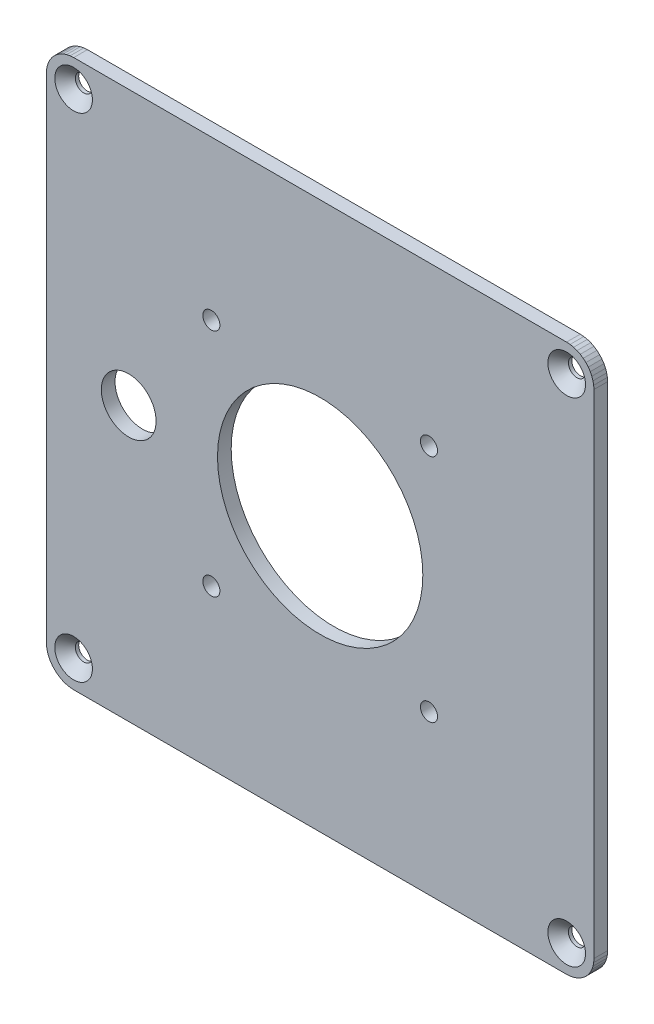
SolidWorks part; units mm, degrees
ref_plane "Front Plane" through (0, 0, 0) normal (0, 0, 1) x (1, 0, 0)
ref_plane "Top Plane" through (0, 0, 0) normal (0, 1, 0) x (1, 0, 0)
ref_plane "Right Plane" through (0, 0, 0) normal (1, 0, 0) x (0, 0, -1)
ref_plane "Plane1" through (0, 0, 196.7768) normal (0, 0, 1) x (1, 0, 0)
sketch "Sketch1" plane through (0, 0, 196.7768) normal (0, 0, 1) x (1, 0, 0)
  line L0 (-40, -36) -> (-39.9658, -36.5221)
  line L1 (-39.9658, -36.5221) -> (-39.8637, -37.0353)
  line L2 (-39.8637, -37.0353) -> (-39.6955, -37.5307)
  line L3 (-39.6955, -37.5307) -> (-39.4641, -38)
  line L4 (-39.4641, -38) -> (-39.1734, -38.435)
  line L5 (-39.1734, -38.435) -> (-38.8284, -38.8284)
  line L6 (-38.8284, -38.8284) -> (-38.435, -39.1734)
  line L7 (-38.435, -39.1734) -> (-38, -39.4641)
  line L8 (-38, -39.4641) -> (-37.5307, -39.6955)
  line L9 (-37.5307, -39.6955) -> (-37.0353, -39.8637)
  line L10 (-37.0353, -39.8637) -> (-36.5221, -39.9658)
  line L11 (-36.5221, -39.9658) -> (-36, -40)
  line L12 (-36, -40) -> (36, -40)
  line L13 (36, -40) -> (36.5221, -39.9658)
  line L14 (36.5221, -39.9658) -> (37.0353, -39.8637)
  line L15 (37.0353, -39.8637) -> (37.5307, -39.6955)
  line L16 (37.5307, -39.6955) -> (38, -39.4641)
  line L17 (38, -39.4641) -> (38.435, -39.1734)
  line L18 (38.435, -39.1734) -> (38.8284, -38.8284)
  line L19 (38.8284, -38.8284) -> (39.1734, -38.435)
  line L20 (39.1734, -38.435) -> (39.4641, -38)
  line L21 (39.4641, -38) -> (39.6955, -37.5307)
  line L22 (39.6955, -37.5307) -> (39.8637, -37.0353)
  line L23 (39.8637, -37.0353) -> (39.9658, -36.5221)
  line L24 (39.9658, -36.5221) -> (40, -36)
  line L25 (40, -36) -> (40, 36)
  line L26 (40, 36) -> (39.9658, 36.5221)
  line L27 (39.9658, 36.5221) -> (39.8637, 37.0353)
  line L28 (39.8637, 37.0353) -> (39.6955, 37.5307)
  line L29 (39.6955, 37.5307) -> (39.4641, 38)
  line L30 (39.4641, 38) -> (39.1734, 38.435)
  line L31 (39.1734, 38.435) -> (38.8284, 38.8284)
  line L32 (38.8284, 38.8284) -> (38.435, 39.1734)
  line L33 (38.435, 39.1734) -> (38, 39.4641)
  line L34 (38, 39.4641) -> (37.5307, 39.6955)
  line L35 (37.5307, 39.6955) -> (37.0353, 39.8637)
  line L36 (37.0353, 39.8637) -> (36.5221, 39.9658)
  line L37 (36.5221, 39.9658) -> (36, 40)
  line L38 (36, 40) -> (-36, 40)
  line L39 (-36, 40) -> (-36.5221, 39.9658)
  line L40 (-36.5221, 39.9658) -> (-37.0353, 39.8637)
  line L41 (-37.0353, 39.8637) -> (-37.5307, 39.6955)
  line L42 (-37.5307, 39.6955) -> (-38, 39.4641)
  line L43 (-38, 39.4641) -> (-38.435, 39.1734)
  line L44 (-38.435, 39.1734) -> (-38.8284, 38.8284)
  line L45 (-38.8284, 38.8284) -> (-39.1734, 38.435)
  line L46 (-39.1734, 38.435) -> (-39.4641, 38)
  line L47 (-39.4641, 38) -> (-39.6955, 37.5307)
  line L48 (-39.6955, 37.5307) -> (-39.8637, 37.0353)
  line L49 (-39.8637, 37.0353) -> (-39.9658, 36.5221)
  line L50 (-39.9658, 36.5221) -> (-40, 36)
  line L51 (-40, 36) -> (-40, -36)
  line L52 (-37.4489, -36.3882) -> (-37.5, -36)
  line L53 (-37.5, -36) -> (-37.4489, -35.6118)
  line L54 (-37.4489, -35.6118) -> (-37.299, -35.25)
  line L55 (-37.299, -35.25) -> (-37.0607, -34.9393)
  line L56 (-37.0607, -34.9393) -> (-36.75, -34.701)
  line L57 (-36.75, -34.701) -> (-36.3882, -34.5511)
  line L58 (-36.3882, -34.5511) -> (-36, -34.5)
  line L59 (-36, -34.5) -> (-35.6118, -34.5511)
  line L60 (-35.6118, -34.5511) -> (-35.25, -34.701)
  line L61 (-35.25, -34.701) -> (-34.9393, -34.9393)
  line L62 (-34.9393, -34.9393) -> (-34.701, -35.25)
  line L63 (-34.701, -35.25) -> (-34.5511, -35.6118)
  line L64 (-34.5511, -35.6118) -> (-34.5, -36)
  line L65 (-34.5, -36) -> (-34.5511, -36.3882)
  line L66 (-34.5511, -36.3882) -> (-34.701, -36.75)
  line L67 (-34.701, -36.75) -> (-34.9393, -37.0607)
  line L68 (-34.9393, -37.0607) -> (-35.25, -37.299)
  line L69 (-35.25, -37.299) -> (-35.6118, -37.4489)
  line L70 (-35.6118, -37.4489) -> (-36, -37.5)
  line L71 (-36, -37.5) -> (-36.3882, -37.4489)
  line L72 (-36.3882, -37.4489) -> (-36.75, -37.299)
  line L73 (-36.75, -37.299) -> (-37.0607, -37.0607)
  line L74 (-37.0607, -37.0607) -> (-37.299, -36.75)
  line L75 (-37.299, -36.75) -> (-37.4489, -36.3882)
  line L76 (-37.4489, 35.6118) -> (-37.5, 36)
  line L77 (-37.5, 36) -> (-37.4489, 36.3882)
  line L78 (-37.4489, 36.3882) -> (-37.299, 36.75)
  line L79 (-37.299, 36.75) -> (-37.0607, 37.0607)
  line L80 (-37.0607, 37.0607) -> (-36.75, 37.299)
  line L81 (-36.75, 37.299) -> (-36.3882, 37.4489)
  line L82 (-36.3882, 37.4489) -> (-36, 37.5)
  line L83 (-36, 37.5) -> (-35.6118, 37.4489)
  line L84 (-35.6118, 37.4489) -> (-35.25, 37.299)
  line L85 (-35.25, 37.299) -> (-34.9393, 37.0607)
  line L86 (-34.9393, 37.0607) -> (-34.701, 36.75)
  line L87 (-34.701, 36.75) -> (-34.5511, 36.3882)
  line L88 (-34.5511, 36.3882) -> (-34.5, 36)
  line L89 (-34.5, 36) -> (-34.5511, 35.6118)
  line L90 (-34.5511, 35.6118) -> (-34.701, 35.25)
  line L91 (-34.701, 35.25) -> (-34.9393, 34.9393)
  line L92 (-34.9393, 34.9393) -> (-35.25, 34.701)
  line L93 (-35.25, 34.701) -> (-35.6118, 34.5511)
  line L94 (-35.6118, 34.5511) -> (-36, 34.5)
  line L95 (-36, 34.5) -> (-36.3882, 34.5511)
  line L96 (-36.3882, 34.5511) -> (-36.75, 34.701)
  line L97 (-36.75, 34.701) -> (-37.0607, 34.9393)
  line L98 (-37.0607, 34.9393) -> (-37.299, 35.25)
  line L99 (-37.299, 35.25) -> (-37.4489, 35.6118)
  line L100 (34.7878, -36.8835) -> (34.6004, -36.5397)
  line L101 (34.6004, -36.5397) -> (34.5085, -36.1591)
  line L102 (34.5085, -36.1591) -> (34.5181, -35.7676)
  line L103 (34.5181, -35.7676) -> (34.6288, -35.392)
  line L104 (34.6288, -35.392) -> (34.8329, -35.0578)
  line L105 (34.8329, -35.0578) -> (35.1165, -34.7878)
  line L106 (35.1165, -34.7878) -> (35.4603, -34.6004)
  line L107 (35.4603, -34.6004) -> (35.8409, -34.5085)
  line L108 (35.8409, -34.5085) -> (36.2324, -34.5181)
  line L109 (36.2324, -34.5181) -> (36.608, -34.6288)
  line L110 (36.608, -34.6288) -> (36.9422, -34.8329)
  line L111 (36.9422, -34.8329) -> (37.2122, -35.1165)
  line L112 (37.2122, -35.1165) -> (37.3996, -35.4603)
  line L113 (37.3996, -35.4603) -> (37.4915, -35.8409)
  line L114 (37.4915, -35.8409) -> (37.4819, -36.2324)
  line L115 (37.4819, -36.2324) -> (37.3713, -36.6081)
  line L116 (37.3713, -36.6081) -> (37.1672, -36.9422)
  line L117 (37.1672, -36.9422) -> (36.8835, -37.2122)
  line L118 (36.8835, -37.2122) -> (36.5397, -37.3996)
  line L119 (36.5397, -37.3996) -> (36.1591, -37.4915)
  line L120 (36.1591, -37.4915) -> (36, -37.4876)
  line L121 (36, -37.4876) -> (35.7676, -37.4819)
  line L122 (35.7676, -37.4819) -> (35.392, -37.3712)
  line L123 (35.392, -37.3712) -> (35.0578, -37.1671)
  line L124 (35.0578, -37.1671) -> (34.7878, -36.8835)
  line L125 (34.5511, 35.6118) -> (34.5, 36)
  line L126 (34.5, 36) -> (34.5511, 36.3882)
  line L127 (34.5511, 36.3882) -> (34.701, 36.75)
  line L128 (34.701, 36.75) -> (34.9393, 37.0607)
  line L129 (34.9393, 37.0607) -> (35.25, 37.299)
  line L130 (35.25, 37.299) -> (35.6118, 37.4489)
  line L131 (35.6118, 37.4489) -> (36, 37.5)
  line L132 (36, 37.5) -> (36.3882, 37.4489)
  line L133 (36.3882, 37.4489) -> (36.75, 37.299)
  line L134 (36.75, 37.299) -> (37.0607, 37.0607)
  line L135 (37.0607, 37.0607) -> (37.299, 36.75)
  line L136 (37.299, 36.75) -> (37.4489, 36.3882)
  line L137 (37.4489, 36.3882) -> (37.5, 36)
  line L138 (37.5, 36) -> (37.4489, 35.6118)
  line L139 (37.4489, 35.6118) -> (37.299, 35.25)
  line L140 (37.299, 35.25) -> (37.0607, 34.9393)
  line L141 (37.0607, 34.9393) -> (36.75, 34.701)
  line L142 (36.75, 34.701) -> (36.3882, 34.5511)
  line L143 (36.3882, 34.5511) -> (36, 34.5)
  line L144 (36, 34.5) -> (35.6118, 34.5511)
  line L145 (35.6118, 34.5511) -> (35.25, 34.701)
  line L146 (35.25, 34.701) -> (34.9393, 34.9393)
  line L147 (34.9393, 34.9393) -> (34.701, 35.25)
  line L148 (34.701, 35.25) -> (34.5511, 35.6118)
extrude "Boss-Extrude1" add sketch "Sketch1" against normal blind 2
sketch "Sketch2" plane through (0, 0, 196.7768) normal (0, 0, 1) x (1, 0, 0)
  circle A0 centre (0, 0) radius 15
  dimension "D1" = 30
extrude "Cut-Extrude1" cut sketch "Sketch2" against normal through all both and the other way through all
sketch "Sketch3" plane through (0, 0, 196.7768) normal (0, 0, 1) x (1, 0, 0)
  circle A0 centre (-27.9726, 0) radius 4
  dimension "D1" = 8
extrude "Cut-Extrude2" cut sketch "Sketch3" against normal blind 10
sketch "Sketch4" plane through (0, 0, 196.7768) normal (0, 0, 1) x (1, 0, 0)
  line L0 (15, 0) -> (-15, 0) construction
  line L1 (-15, 0) -> (0, 0) construction
  line L2 (0, 0) -> (0, 15) construction
  circle A0 centre (15.8981, 16.8222) radius 1.25
  circle A1 centre (0, 0) radius 15 construction
  circle A2 centre (-15.8981, 16.8222) radius 1.25
  circle A3 centre (-15.8981, -16.8222) radius 1.25
  circle A4 centre (15.8981, -16.8222) radius 1.25
  dimension "D1" = 2.5
  dimension "D2" = 2.5
extrude "Cut-Extrude3" cut sketch "Sketch4" against normal blind 10
sketch "Sketch5" plane through (0, 0, 196.7768) normal (0, 0, 1) x (1, 0, 0)
  line L0 (36.0129, -37.4879) -> (36.0367, -34.5133) construction
  line L1 (35.7676, -37.4819) -> (36.1591, -37.4915) construction
  line L2 (36.2324, -34.5181) -> (35.8409, -34.5085) construction
  line L3 (36.0367, -34.5133) -> (36.0248, -36.0006) construction
  line L4 (0, 0) -> (0, -40) construction
  line L5 (-36, -40) -> (36, -40) construction
  line L6 (0, -40) -> (0, 0) construction
  line L7 (0, 0) -> (40, 0) construction
  line L8 (40, -36) -> (40, 36) construction
  line L9 (-36.0367, -34.5133) -> (-36.0248, -36.0006) construction
  line L10 (-36.0129, -37.4879) -> (-36.0367, -34.5133) construction
  line L11 (-36.0129, 37.4879) -> (-36.0367, 34.5133) construction
  line L12 (-36.0367, 34.5133) -> (-36.0248, 36.0006) construction
  line L13 (36.0367, 34.5133) -> (36.0248, 36.0006) construction
  line L14 (36.0129, 37.4879) -> (36.0367, 34.5133) construction
  circle A0 centre (36.0248, -36.0006) radius 2
  circle A1 centre (-36.0248, -36.0006) radius 2
  circle A2 centre (-36.0248, 36.0006) radius 2
  circle A3 centre (36.0248, 36.0006) radius 2
  dimension "D1" = 4
extrude "Cut-Extrude4" cut sketch "Sketch5" against normal blind 10
other "Move Face1" face at (34.0248, 36.0006, 196.7768) face at (-34.0248, 36.0006, 196.7768) face at (-38.0248, -36.0006, 196.7768) face at (38.0248, -36.0006, 196.7768) parameters "D1"=0.75
chamfer "Chamfer1" distance 1.5 angle 45 4 edges at (37.2748, -36.0006, 196.7768) (-34.7748, -36.0006, 196.7768) (-34.7748, 36.0006, 196.7768) (37.2748, 36.0006, 196.7768)
